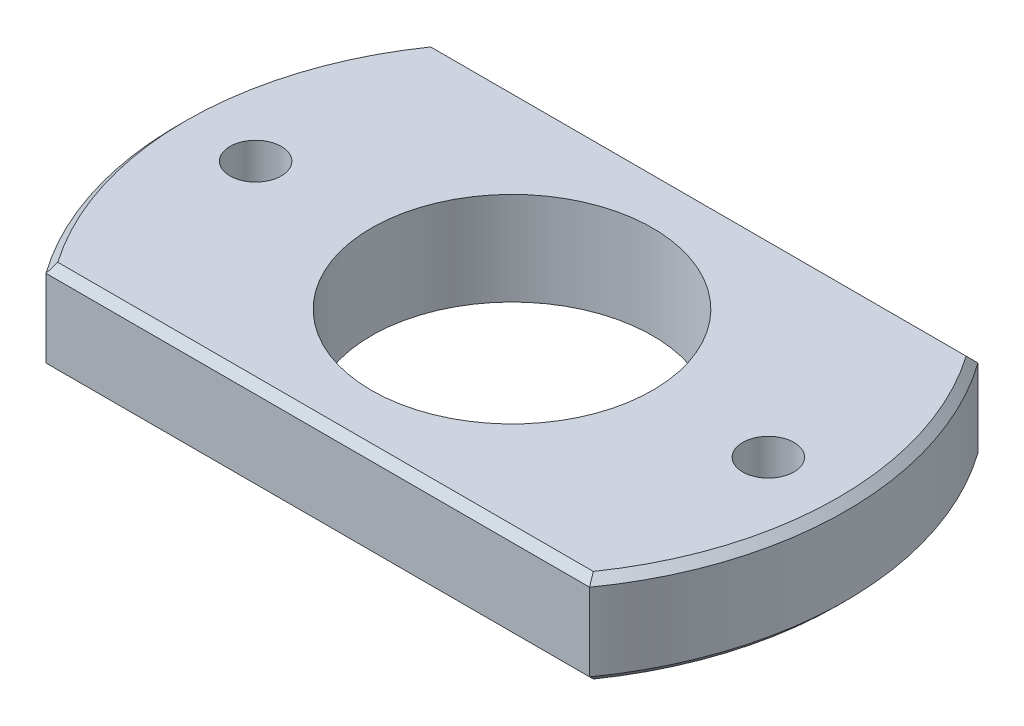
SolidWorks part; units mm, degrees
material "SUS 304"
ref_plane "前视基准面" through (0, 0, 0) normal (0, 0, 1) x (1, 0, 0)
ref_plane "上视基准面" through (0, 0, 0) normal (0, 1, 0) x (1, 0, 0)
ref_plane "右视基准面" through (0, 0, 0) normal (1, 0, 0) x (0, 0, -1)
sketch "草图1" plane through (0, 0, 0) normal (0, 1, 0) x (1, 0, 0)
  circle A0 centre (0, 0) radius 21.5
  dimension "D1" = 43
extrude "凸台-拉伸1" add sketch "草图1" along normal blind 6
hole_wizard "M4 螺纹孔1" positions "草图4" profile "草图3" tap size "M4" standard "GB" end condition through all
sketch "草图4" plane through (0, 6, 0) normal (0, 1, 0) x (1, 0, 0)
  line L0 (-16.5, 0) -> (16.5, 0) construction
  point P0 (-16.5, 0)
  point P2 (16.5, 0)
  dimension "D1" = 33
sketch "草图3" plane through (-16.5, 6, 0) normal (1, 0, 0) x (0, 0, 1)
  line L0 (0, 0) -> (0, 6)
  line L1 (0, 6) -> (1.65, 6)
  line L2 (1.65, 6) -> (1.65, 0)
  line L5 (1.65, 0) -> (0, 0)
  line L11 (0, -6.35) -> (0, 107.95) construction
  dimension "通孔螺纹孔钻头直径" = 3.3
  dimension "通孔螺纹孔钻头深度" = 6
cosmetic thread "孔螺蚊线1" parameters "D2"=4
cosmetic thread "孔螺蚊线2" parameters "D2"=4
sketch "草图5" plane through (0, 6, 0) normal (0, 1, 0) x (1, 0, 0)
  line L0 (0, 0) -> (21.5, 0) construction
  line L1 (-45.3063, 35.6655) -> (34.8819, 35.6655)
  line L2 (-45.3063, 35.6655) -> (-45.3063, 12.5)
  line L3 (-45.3063, 12.5) -> (34.8819, 12.5)
  line L4 (34.8819, 35.6655) -> (34.8819, 12.5)
  line L5 (-45.3063, 35.6655) -> (34.8819, 12.5) construction
  line L6 (-45.3063, 12.5) -> (34.8819, 35.6655) construction
  line L7 (94.7214, -39.4076) -> (-51.7214, -39.4076)
  line L8 (94.7214, -39.4076) -> (94.7214, -12.5)
  line L9 (94.7214, -12.5) -> (-51.7214, -12.5)
  line L10 (-51.7214, -39.4076) -> (-51.7214, -12.5)
  line L11 (94.7214, -39.4076) -> (-51.7214, -12.5) construction
  line L12 (94.7214, -12.5) -> (-51.7214, -39.4076) construction
  circle A0 centre (0, 0) radius 21.5 construction
  point P0 (-5.2122, 24.0827)
  point P5 (21.5, -25.9538)
  dimension "D1" = 25
extrude "切除-拉伸1" cut sketch "草图5" against normal through all
hole_wizard "M20 螺纹孔2" positions "草图9" profile "草图8" tap size "M20" standard "GB" end condition through all
sketch "草图9" plane through (0, 6, 0) normal (0, 1, 0) x (1, 0, 0)
  point P0 (0, 0)
sketch "草图8" plane through (0, 6, 0) normal (1, 0, 0) x (0, 0, 1)
  line L0 (0, 0) -> (0, 6)
  line L1 (0, 6) -> (9.05, 6)
  line L2 (9.05, 6) -> (9.05, 0)
  line L5 (9.05, 0) -> (0, 0)
  line L11 (0, -6.35) -> (0, 107.95) construction
  dimension "通孔螺纹孔钻头直径" = 18.1
  dimension "通孔螺纹孔钻头深度" = 6
cosmetic thread "孔螺蚊线3" parameters "D2"=20
chamfer "倒角1" distance 0.5 angle 45 8 edges at (21.5, 0, 0) (-21.5, 0, 0) (0, 0, -12.5) (0, 0, 12.5) (21.5, 6, 0) (-21.5, 6, 0) (0, 6, -12.5) (0, 6, 12.5)
